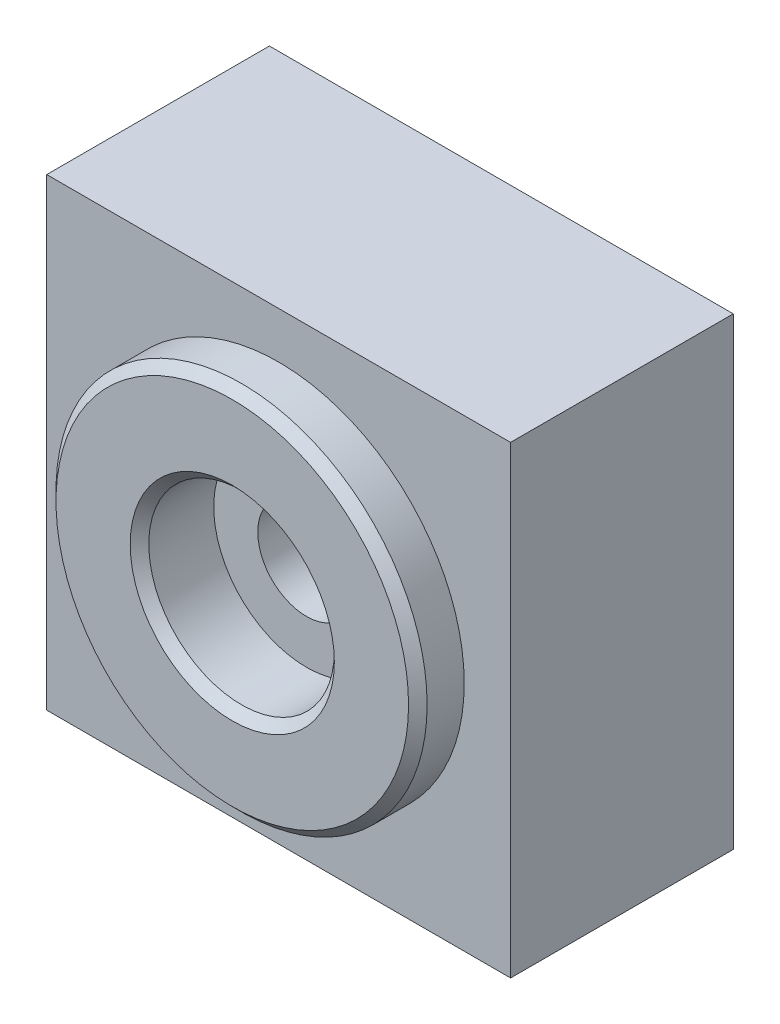
SolidWorks part; units mm, degrees
material "1023 碳钢板 (SS)"
ref_plane "前视基准面" through (0, 0, 0) normal (0, 0, 1) x (1, 0, 0)
ref_plane "上视基准面" through (0, 0, 0) normal (0, 1, 0) x (1, 0, 0)
ref_plane "右视基准面" through (0, 0, 0) normal (1, 0, 0) x (0, 0, -1)
sketch "草图1" plane through (0, 0, 0) normal (0, 0, 1) x (1, 0, 0)
  line L1 (-25, 25) -> (25, 25)
  line L2 (-25, 25) -> (-25, -25)
  line L3 (-25, -25) -> (25, -25)
  line L4 (25, 25) -> (25, -25)
  line L5 (-25, 25) -> (25, -25) construction
  line L6 (-25, -25) -> (25, 25) construction
  point P0 (0, 0)
  dimension "D1" = 50
  dimension "D2" = 50
extrude "凸台-拉伸1" add sketch "草图1" along normal blind 29
sketch "草图3" plane through (0, 0, 29) normal (0, 0, 1) x (1, 0, 0)
  circle A0 centre (0, 0) radius 10
  dimension "D1" = 20
extrude "切除-拉伸1" cut sketch "草图3" against normal blind 8
sketch "草图4" plane through (0, 0, 0) normal (0, 0, -1) x (-1, 0, 0)
  circle A0 centre (0, 0) radius 5.25
  dimension "D1" = 10.5
extrude "切除-拉伸2" cut sketch "草图4" against normal blind 21
chamfer "倒角1" distance 1 angle 45 1 edges at (10, 0, 29)
sketch "草图5" plane through (0, 0, 29) normal (0, 0, 1) x (1, 0, 0)
  circle A0 centre (0, 0) radius 20
  dimension "D1" = 40
extrude "切除-拉伸3" cut sketch "草图5" against normal blind 5 flip side to cut
chamfer "倒角2" distance 1 angle 45 1 edges at (20, 0, 29)
